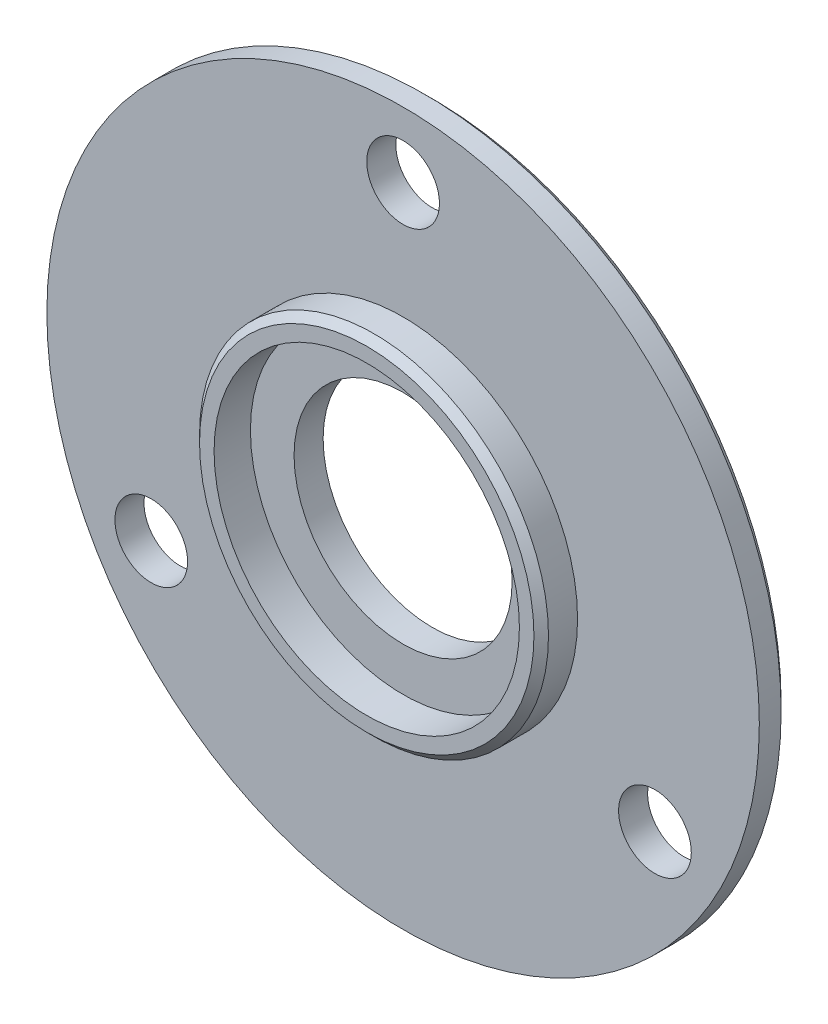
SolidWorks part; units mm, degrees
ref_plane "Front Plane" through (0, 0, 0) normal (0, 0, 1) x (1, 0, 0)
ref_plane "Top Plane" through (0, 0, 0) normal (0, 1, 0) x (1, 0, 0)
ref_plane "Right Plane" through (0, 0, 0) normal (1, 0, 0) x (0, 0, -1)
other "Configuration Table"
sketch "Sketch1" plane through (0, 0, 0) normal (0, 0, 1) x (1, 0, 0)
  circle A0 centre (0, 0) radius 24.5
  dimension "D1" = 49
extrude "Boss-Extrude1" add sketch "Sketch1" along normal blind 2
sketch "Sketch2" plane through (0, 0, 2) normal (0, 0, 1) x (1, 0, 0)
  circle A0 centre (0, 0) radius 12
  dimension "D1" = 24
extrude "Boss-Extrude2" add sketch "Sketch2" along normal blind 2.5
sketch "Sketch3" plane through (0, 0, 2) normal (0, 0, 1) x (1, 0, 0)
  circle A0 centre (0, 0) radius 10.5
  dimension "D1" = 21
extrude "Cut-Extrude1" cut sketch "Sketch3" against normal blind 2.5 from surface at 2.5 starting at face at (12, 0, 4.5)
sketch "Sketch4" plane through (0, 0, 2) normal (0, 0, 1) x (1, 0, 0)
  circle A0 centre (0, 0) radius 7.5
  dimension "D1" = 15
extrude "Cut-Extrude2" cut sketch "Sketch4" against normal blind 2.5
sketch "Sketch5" plane through (0, 0, 2) normal (0, 0, 1) x (1, 0, 0)
  circle A0 centre (0, 0) radius 20 construction
  circle A1 centre (0, 20) radius 2.5
  circle A2 centre (17.3205, -10) radius 2.5
  circle A3 centre (-17.3205, -10) radius 2.5
  point P12 (0, 0)
  dimension "D1" = 40
  dimension "D2" = 5
  dimension "D3" = 3
extrude "Cut-Extrude3" cut sketch "Sketch5" against normal blind 2.5
chamfer "Chamfer1" distance 0.5 angle 45 2 edges at (24.5, 0, 0) (12, 0, 4.5)
